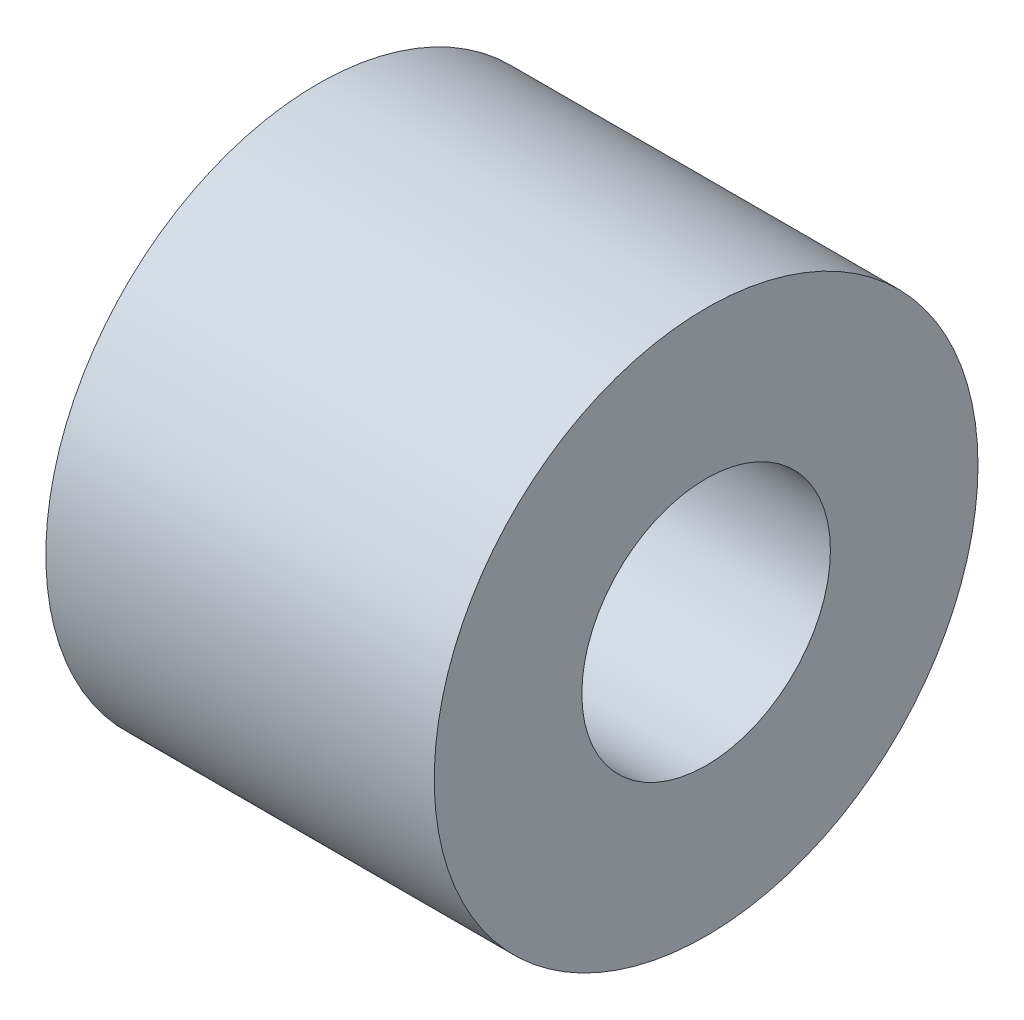
from build123d import *

# Parameters (mm, degrees)
SKETCH_1_R      = 3.5
SKETCH_1_R_2    = 1.6
EXTRUDE_1_DEPTH = 5


with BuildPart() as part:
    # 草图1 → 凸台-拉伸1 (new body)
    with BuildSketch(Plane(origin=(0, 0, 0), x_dir=(0, 0, -1), z_dir=(1, 0, 0))):
        Circle(SKETCH_1_R)
        Circle(SKETCH_1_R_2, mode=Mode.SUBTRACT)
    extrude(amount=EXTRUDE_1_DEPTH)


solid = part.part
